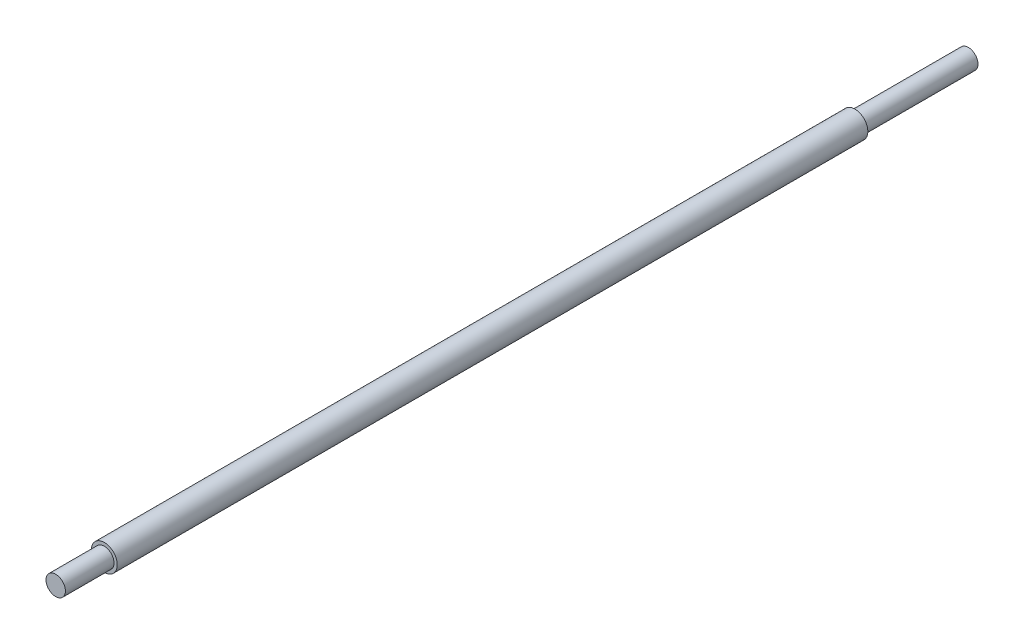
from build123d import *

# Parameters (mm, degrees)
SKETCH1_R           = 8
BOSS_EXTRUDE1_DEPTH = 231.7
SKETCH2_R           = 6
BOSS_EXTRUDE2_DEPTH = 30
BOSS_EXTRUDE3_START = 70
SKETCH4_R           = 6
BOSS_EXTRUDE3_DEPTH = 70


with BuildPart() as part:
    # Sketch1 → Boss-Extrude1 (new, symmetric)
    with BuildSketch(Plane.XY):
        with Locations(Location((0, 0, 0), (0, 0, 180))):
            Circle(SKETCH1_R)
    extrude(amount=BOSS_EXTRUDE1_DEPTH, both=True)

    # Sketch2 → Boss-Extrude2 (add)
    with BuildSketch(Plane.XY.offset(231.7)):
        Circle(SKETCH2_R)
    extrude(amount=BOSS_EXTRUDE2_DEPTH)

    # Sketch4 → Boss-Extrude3 (add)
    with BuildSketch(Plane(origin=(0, 0, -231.7), x_dir=(-1, 0, 0), z_dir=(0, 0, -1)).offset(BOSS_EXTRUDE3_START)):
        with Locations(Location((0, 0, 0), (0, 0, 180))):
            Circle(SKETCH4_R)
    extrude(amount=-BOSS_EXTRUDE3_DEPTH)


solid = part.part
